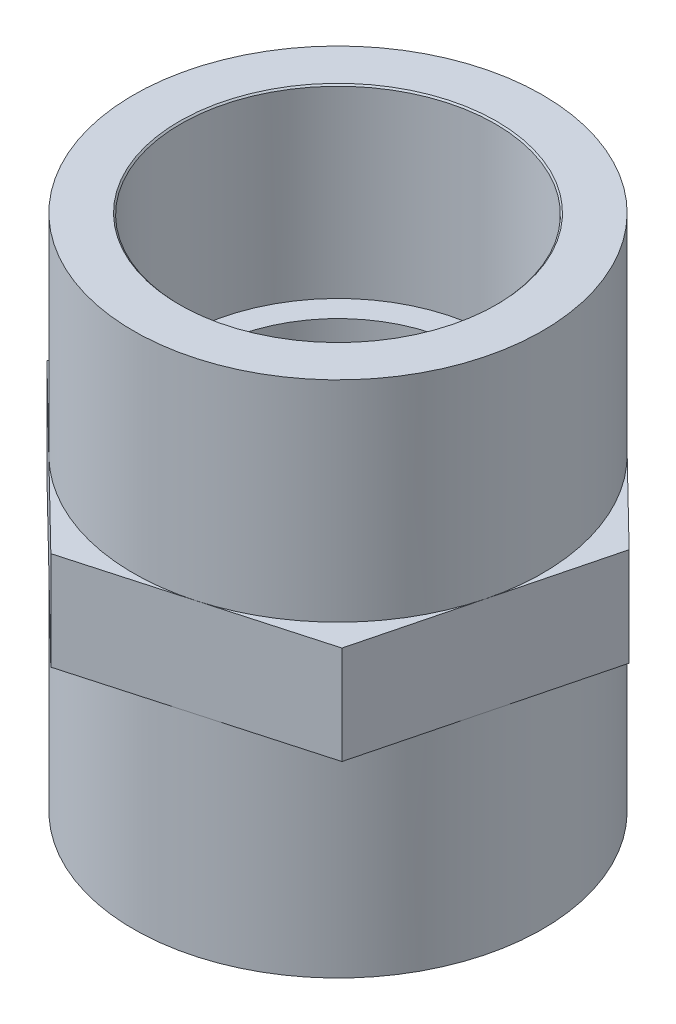
from build123d import *

# Parameters (mm, degrees)
SKETCH_3_W          = 2.4
SKETCH_3_H          = 3.7
EXTRUDE_1_DEPTH     = 5
CUT_EXTRUDE_START   = -10
SKETCH_5_R          = 16
CUT_EXTRUDE_1_DEPTH = 10
SKETCH_6_R          = 17.5
SKETCH_6_R_2        = 13.5
EXTRUDE_2_DEPTH     = 7.5


with BuildPart() as part:
    # 草图2 → Revolve 1 (revolve)
    with BuildSketch(Plane.XY, mode=Mode.PRIVATE) as revolve_1_sk:
        Polygon((-16, 26.2), (-16, -26.35), (-20.8, -26.35), (-20.8, 26.35), (-16.15, 26.35), align=None)
    revolve(revolve_1_sk.sketch.rotate(Axis((0, -26.35, 0), (0, 1, 0)), 270), axis=Axis((0, -26.35, 0), (0, 1, 0)))

    # 草图3 → Revolve 1 2 (revolve)
    with BuildSketch(Plane.XY, mode=Mode.PRIVATE) as revolve_1_2_sk:
        with Locations((-14.8, 1.85)):
            Rectangle(SKETCH_3_W, SKETCH_3_H)
    revolve(revolve_1_2_sk.sketch.rotate(Axis((0, -26.35, 0), (0, 1, 0)), 270), axis=Axis((0, -26.35, 0), (0, 1, 0)))

    # 草图4 → 凸台-拉伸1 (add, symmetric)
    with BuildSketch(Plane(origin=(0, 0, 0), x_dir=(1, 0, 0), z_dir=(0, 1, 0))):
        Polygon((23.124383018, 6.489702871), (5.94194396, 23.271154576), (-17.182439058, 16.781451705), (-23.124383018, -6.489702871), (-5.94194396, -23.271154576), (17.182439058, -16.781451705), align=None)
    extrude(amount=EXTRUDE_1_DEPTH, both=True)

    # 草图5 → 切除-拉伸1 (cut)
    with BuildSketch(Plane(origin=(0, 5, 0), x_dir=(1, 0, 0), z_dir=(0, 1, 0)).offset(CUT_EXTRUDE_START)):
        with Locations(Location((0, 0, 0), (0, 0, 90))):
            Circle(SKETCH_5_R)
    extrude(amount=CUT_EXTRUDE_1_DEPTH, mode=Mode.SUBTRACT)

    # 草图6 → 凸台-拉伸2 (add, symmetric)
    with BuildSketch(Plane(origin=(0, 0, 0), x_dir=(1, 0, 0), z_dir=(0, 1, 0))):
        Circle(SKETCH_6_R)
        with Locations(Location((0, 0, 0), (0, 0, 270))):
            Circle(SKETCH_6_R_2, mode=Mode.SUBTRACT)
    extrude(amount=EXTRUDE_2_DEPTH, both=True)


solid = part.part
